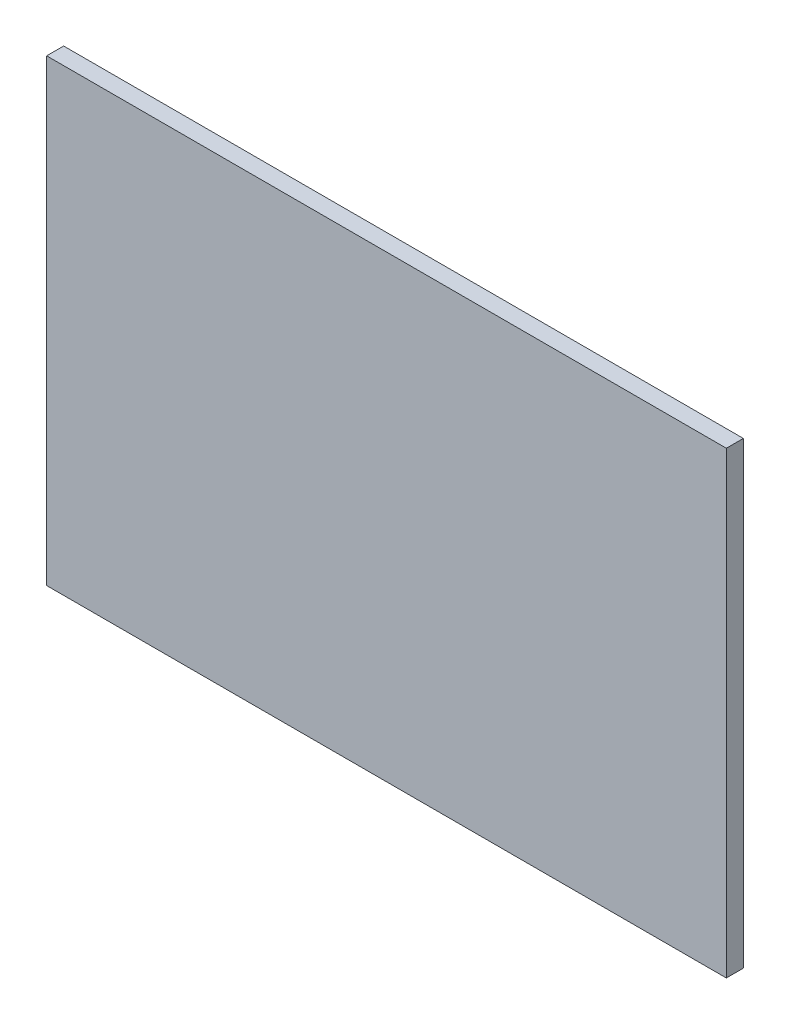
SolidWorks part; units mm, degrees
material "普通碳钢"
ref_plane "Front Plane" through (0, 0, 0) normal (0, 0, 1) x (1, 0, 0)
ref_plane "Top Plane" through (0, 0, 0) normal (0, 1, 0) x (1, 0, 0)
ref_plane "Right Plane" through (0, 0, 0) normal (1, 0, 0) x (0, 0, -1)
sketch "Sketch1" plane through (0, 0, 0) normal (0, 0, 1) x (1, 0, 0)
  line L1 (-200, 135) -> (200, 135)
  line L2 (-200, 135) -> (-200, -135)
  line L3 (-200, -135) -> (200, -135)
  line L4 (200, 135) -> (200, -135)
  dimension "D1" = 270
  dimension "D2" = 400
  dimension "D3" = 135
  dimension "D4" = 200
extrude "Boss-Extrude1" add sketch "Sketch1" along normal mid plane 10
